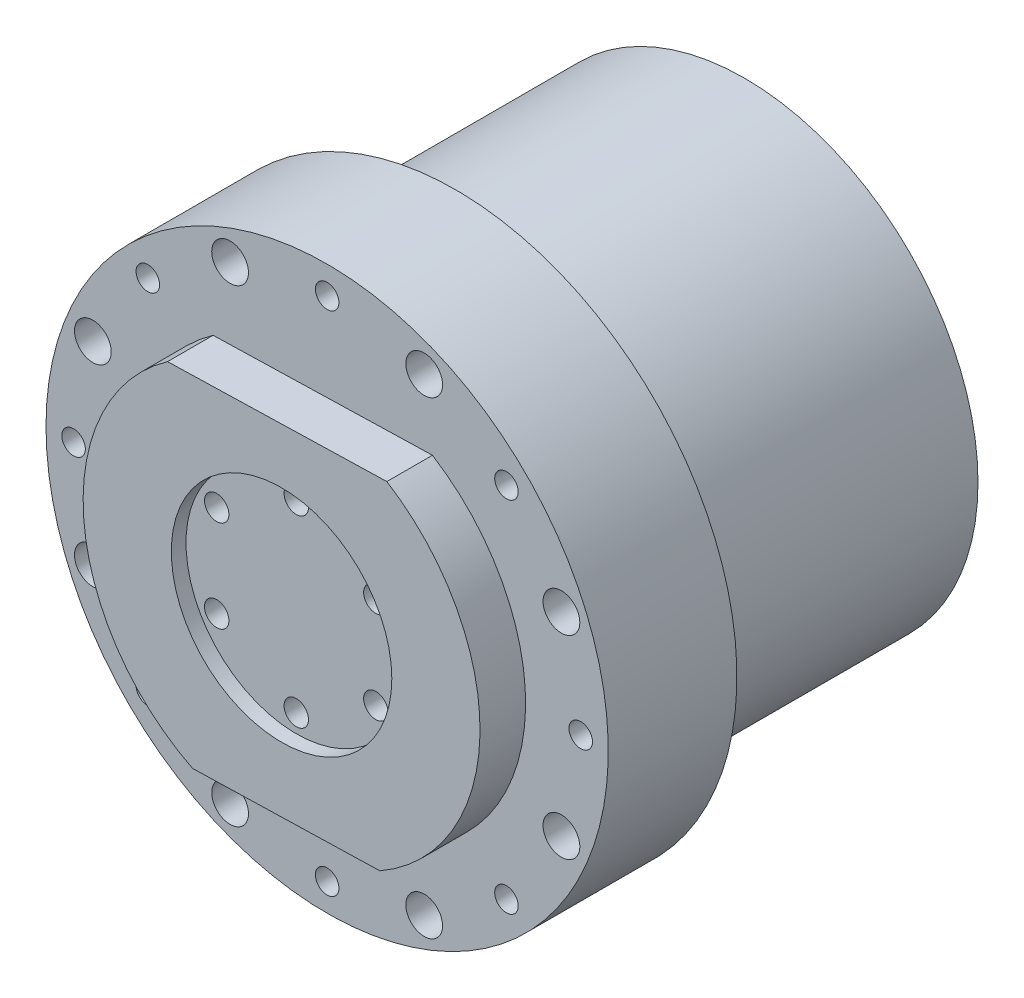
SolidWorks part; units mm, degrees
ref_plane "Front Plane" through (0, 0, 0) normal (0, 0, 1) x (1, 0, 0)
ref_plane "Top Plane" through (0, 0, 0) normal (0, 1, 0) x (1, 0, 0)
ref_plane "Right Plane" through (0, 0, 0) normal (1, 0, 0) x (0, 0, -1)
sketch "Sketch1" plane through (0, 0, 0) normal (0, 0, 1) x (1, 0, 0)
  line L0 (0, 12.5) -> (0, 0) construction
  line L1 (0, 0) -> (7.0092, 12.1402) construction
  line L2 (0, 0) -> (16.5038, 0) construction
  line L3 (-15.5161, 22.0964) -> (14.3253, 22.8864)
  line L4 (-12.1142, -24.1298) -> (13.3739, -23.455)
  arc A0 (-15.5161, 22.0964) -> (-12.1142, -24.1298) centre (0, 0) ccw
  circle A1 centre (0, 0) radius 12.5 construction
  circle A2 centre (0, 12.5) radius 1.66
  circle A3 centre (10.8253, 6.25) radius 1.66
  circle A4 centre (0, -12.5) radius 1.66
  circle A5 centre (10.8253, -6.25) radius 1.66
  circle A6 centre (-10.8253, -6.25) radius 1.66
  circle A7 centre (-10.8253, 6.25) radius 1.66
  arc A8 (13.3739, -23.455) -> (14.3253, 22.8864) centre (0, 0) ccw
  dimension "D1" = 30
  dimension "D2" = 54
  dimension "D3" = 46.3
extrude "Boss-Extrude1" add sketch "Sketch1" along normal blind 6.2
ref_plane "Plane1" through (0, 0, 0) normal (0, 0, -1) x (-1, 0, 0)
sketch "Sketch2" plane through (0, 0, 0) normal (0, 0, -1) x (-1, 0, 0)
  line L0 (0, 34.5) -> (0, 0) construction
  line L1 (0, 0) -> (15.3309, 37.0121) construction
  line L2 (0, 0) -> (29.9174, 29.9174) construction
  line L3 (0, 0) -> (38.5391, 15.9634) construction
  line L4 (0, 0) -> (52.4604, 0) construction
  line L5 (0, 0) -> (31.8738, -13.2026) construction
  circle A0 centre (0, 0) radius 38.25
  circle A1 centre (0, 0) radius 34.5 construction
  circle A2 centre (0, 34.5) radius 1.6
  circle A3 centre (24.3952, 24.3952) radius 1.6
  circle A4 centre (34.5, 0) radius 1.6
  circle A5 centre (24.3952, -24.3952) radius 1.6
  circle A6 centre (0, -34.5) radius 1.6
  circle A7 centre (-24.3952, -24.3952) radius 1.6
  circle A8 centre (-34.5, 0) radius 1.6
  circle A9 centre (-24.3952, 24.3952) radius 1.6
  circle A10 centre (13.2026, 31.8738) radius 2.5
  circle A11 centre (31.8738, 13.2026) radius 2.5
  circle A12 centre (31.8738, -13.2026) radius 2.5
  circle A13 centre (13.2026, -31.8738) radius 2.5
  circle A14 centre (-31.8738, -13.2026) radius 2.5
  circle A15 centre (-31.8738, 13.2026) radius 2.5
  circle A16 centre (-13.2026, 31.8738) radius 2.5
  circle A17 centre (-13.2026, -31.8738) radius 2.5
  dimension "D1" = 22.5
  dimension "D4" = 34.5
  dimension "D5" = 76.5
  dimension "D2" = 45
  dimension "D3" = 22.5
extrude "Boss-Extrude2" add sketch "Sketch2" along normal blind 17.5
ref_plane "Plane2" through (0, 0, -17.5) normal (0, 0, -1) x (-1, 0, 0)
sketch "Sketch3" plane through (0, 0, -17.5) normal (0, 0, -1) x (-1, 0, 0)
  circle A0 centre (0, 0) radius 31.75
extrude "Boss-Extrude3" add sketch "Sketch3" along normal blind 39.3 contours A0
sketch "Sketch4" plane through (0, 0, 6.2) normal (0, 0, 1) x (1, 0, 0)
  circle A0 centre (0, 0) radius 15
  dimension "D1" = 30
extrude "Cut-Extrude1" cut sketch "Sketch4" against normal blind 2
